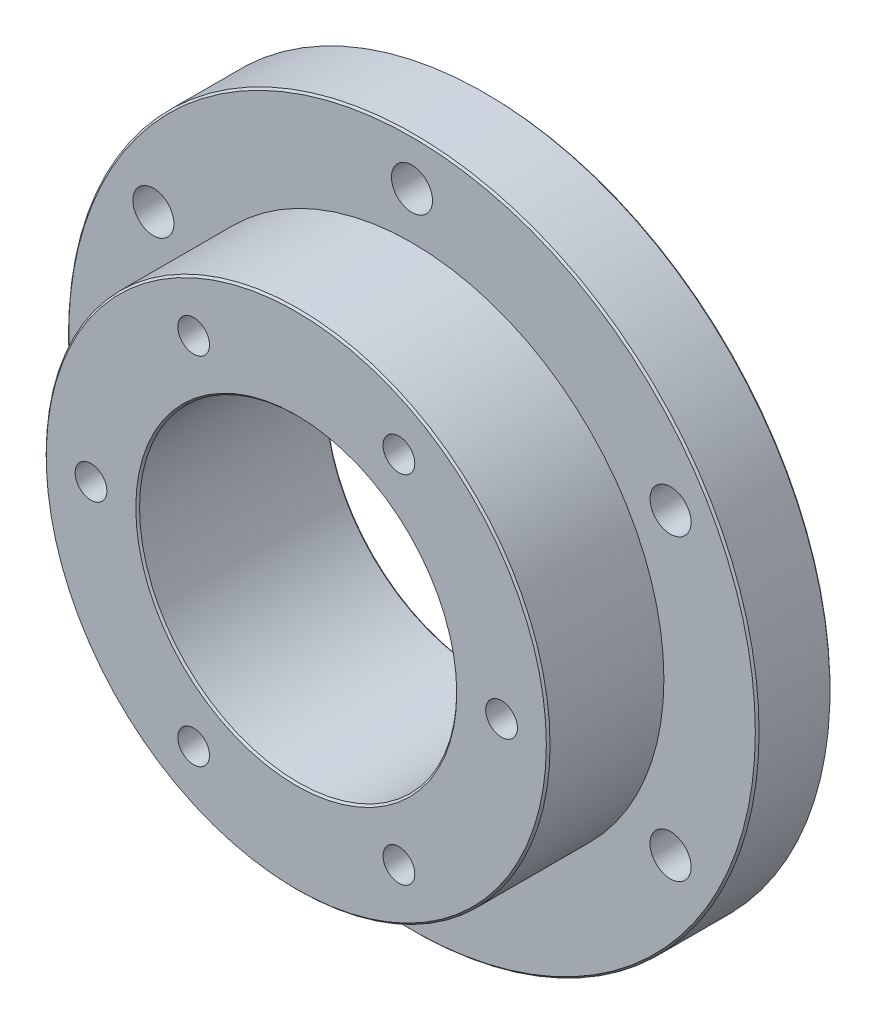
SolidWorks part; units mm, degrees
material "合金钢"
ref_plane "前视基准面" through (0, 0, 0) normal (0, 0, 1) x (1, 0, 0)
ref_plane "上视基准面" through (0, 0, 0) normal (0, 1, 0) x (1, 0, 0)
ref_plane "右视基准面" through (0, 0, 0) normal (1, 0, 0) x (0, 0, -1)
sketch "草图1" plane through (0, 0, 0) normal (0, 1, 0) x (1, 0, 0)
  line L0 (0, 0) -> (0, -85339.322) construction
  line L1 (-42.5, 20) -> (-42.5, -31)
  line L2 (-42.5, -31) -> (-67.5, -31)
  line L3 (-67.5, -31) -> (-67.5, 0)
  line L4 (-67.5, 0) -> (-92.5, 0)
  line L5 (-92.5, 0) -> (-92.5, 20)
  line L6 (-92.5, 20) -> (-42.5, 20)
  dimension "D1" = 85
  dimension "D2" = 25
  dimension "D3" = 51
  dimension "D4" = 20
  dimension "D5" = 25
revolve "旋转1" add sketch "草图1" angle 360 about L0
hole_wizard "打孔尺寸(%根据)内六角圆柱头螺钉的类型1" positions "草图4" profile "草图5" counterbore size "M10" standard "GB" end condition through all
sketch "草图4" plane through (0, 0, -20) normal (0, 0, 1) x (1, 0, 0)
  circle A1 centre (0, 0) radius 92.5 construction
  point P0 (0, -80)
  dimension "D1" = 12.5
sketch "草图5" plane through (0, -80, -20) normal (1, 0, 0) x (0, 1, 0)
  line L0 (0, 0) -> (0, 51)
  line L1 (0, 51) -> (5.5, 51)
  line L3 (5.5, 51) -> (5.5, 11)
  line L4 (5.5, 11) -> (9, 11)
  line L5 (9, 11) -> (9, 0)
  line L7 (9, 0) -> (0, 0)
  line L11 (0, -6.35) -> (0, 107.95) construction
  dimension "通孔孔直径" = 11
  dimension "通孔孔深度" = 51
  dimension "柱形沉头孔直径" = 18
  dimension "柱形沉头孔深度" = 11
pattern_circular "阵列(圆周)1" count 6 over 360 about axis through (0, 0, 0) along (0, 0, 1) of "打孔尺寸(%根据)内六角圆柱头螺钉的类型1"
hole_wizard "M10 螺纹孔1" positions "草图6" profile "草图7" tap size "M10" standard "GB"
sketch "草图6" plane through (0, 0, 31) normal (0, 0, 1) x (1, 0, 0)
  circle A2 centre (0, 0) radius 67.5 construction
  point P0 (-55, 0)
  dimension "D1" = 12.5
sketch "草图7" plane through (-55, 0, 31) normal (1, 0, 0) x (0, -1, 0)
  line L0 (0, 0) -> (0, 27.0537)
  line L1 (0, 27.0537) -> (4.25, 24.5)
  line L2 (4.25, 24.5) -> (4.25, 0)
  line L5 (4.25, 0) -> (0, 0)
  line L10 (0, 27.0537) -> (-4.25, 24.5) construction
  line L11 (0, -6.35) -> (0, 107.95) construction
  dimension "螺纹孔钻头直径" = 8.5
  dimension "螺纹孔钻头深度" = 24.5
  dimension "导头角度" = 118
cosmetic thread "孔螺蚊线1" parameters "D1"=20, "D2"=10
pattern_circular "阵列(圆周)2" count 6 over 360 about axis through (0, 0, 0) along (0, 0, 1) of "M10 螺纹孔1"
chamfer "倒角1" distance 0.5 angle 45 5 edges at (-42.5, 0, -20) (-42.5, 0, 31) (-67.5, 0, 31) (-92.5, 0, 0) (-92.5, 0, -20)
